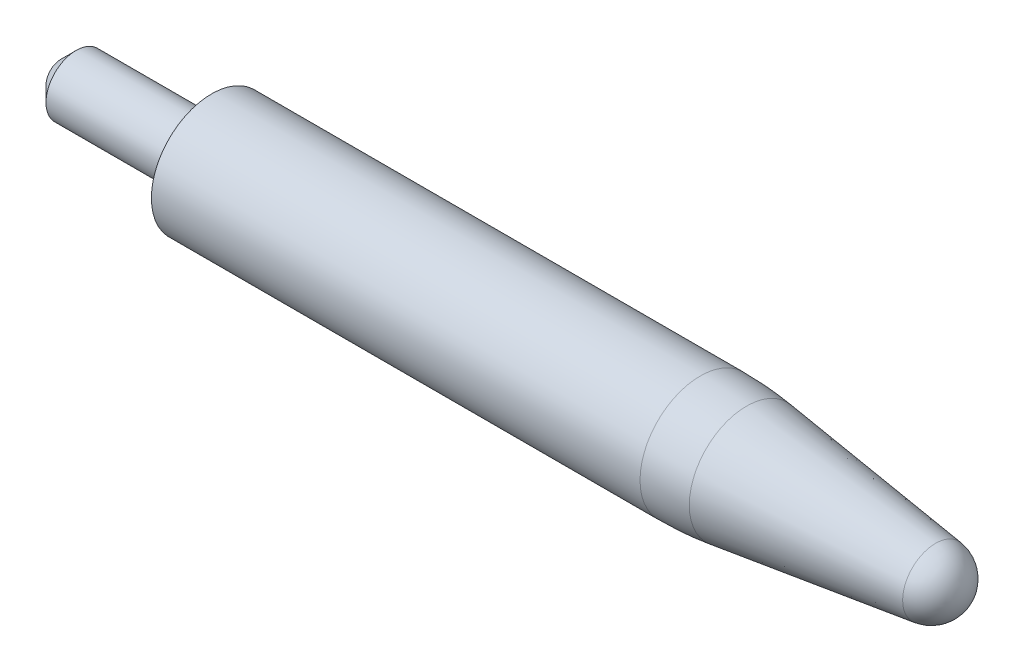
SolidWorks part; units mm, degrees
ref_plane "Front Plane" through (0, 0, 0) normal (0, 0, 1) x (1, 0, 0)
ref_plane "Top Plane" through (0, 0, 0) normal (0, 1, 0) x (1, 0, 0)
ref_plane "Right Plane" through (0, 0, 0) normal (1, 0, 0) x (0, 0, -1)
sketch "Sketch1" plane through (0, 0, 0) normal (0, 0, 1) x (1, 0, 0)
  line L0 (0, 0) -> (96.875, 0) construction
  line L1 (0, 0) -> (0, 2)
  line L2 (0, 2) -> (16.2285, 2)
  line L3 (17, 2) -> (17, 0) construction
  line L4 (17, 0) -> (25, 0) construction
  line L5 (17.7651, 1.9012) -> (24.0409, 1.0909)
  line L6 (0, 0) -> (25, 0)
  arc A0 (25, 0) -> (24.0409, 1.0909) centre (23.9, 0) ccw
  arc A1 (17.7651, 1.9012) -> (16.2285, 2) centre (16.2285, -10) ccw
  dimension "D4" = 2.2
  dimension "D5" = 12
  dimension "D1" = 4
  dimension "D2" = 17
  dimension "D3" = 8
revolve "Revolve1" add sketch "Sketch1" angle 360 about L6
sketch "Sketch2" plane through (0, 0, 0) normal (-1, 0, 0) x (0, 0, 1)
  circle A0 centre (0, 0) radius 1
  dimension "D1" = 2
extrude "Boss-Extrude1" add sketch "Sketch2" along normal blind 5
chamfer "Chamfer1" distance 0.5 angle 45 1 edges at (-5, 0, 1)
equation "\"1\"= \"代号代号\""
equation "\"2\"= \"名称代号\""
